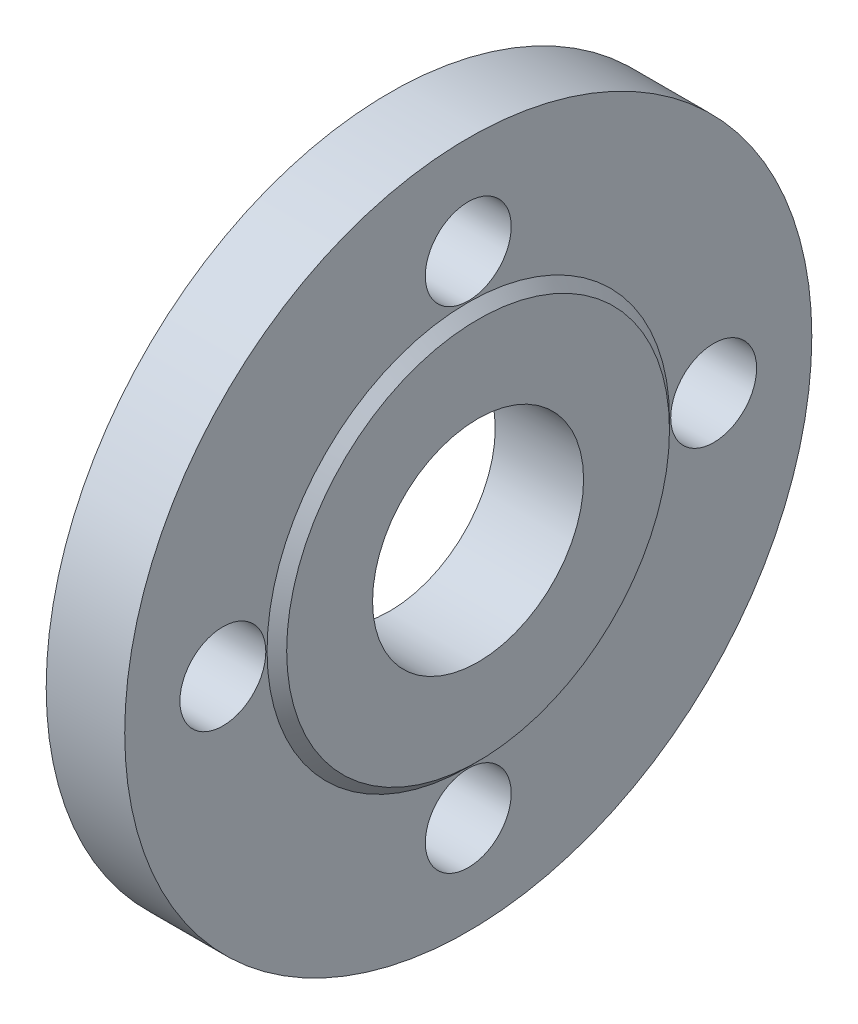
from build123d import *

# Parameters (mm, degrees)
CUT_EXTRUDE_1_DEPTH      = 101.279609094
CUT_EXTRUDE_1_DEPTH_BACK = 101.279609094
SKETCH_2_R               = 8.75


with BuildPart() as part:
    # 草图1 → 旋转1 (revolve)
    with BuildSketch(Plane(origin=(0, 0, 0), x_dir=(1, 0, 0), z_dir=(0, 1, 0)), mode=Mode.PRIVATE) as revolve_1_sk:
        Polygon((0, 21.5), (0, 70), (16, 70), (16, 41), (18, 39), (18, 21.5), align=None)
    revolve(revolve_1_sk.sketch.rotate(Axis((0, 0, 0), (1, 0, 0)), 180), axis=Axis((0, 0, 0), (1, 0, 0)))

    # 草图2 → 切除-拉伸1 (cut, two sides: drawn at the far end of the back side and taken through both)
    with BuildSketch(Plane(origin=(16, 0, 0), x_dir=(0, 0, -1), z_dir=(1, 0, 0)).offset(-CUT_EXTRUDE_1_DEPTH_BACK)):
        with Locations((0, 50)):
            Circle(SKETCH_2_R)
        with Locations((50, 0)):
            Circle(SKETCH_2_R)
        with Locations((0, -50)):
            Circle(SKETCH_2_R)
        with Locations((-50, 0)):
            Circle(SKETCH_2_R)
    extrude(amount=CUT_EXTRUDE_1_DEPTH + CUT_EXTRUDE_1_DEPTH_BACK, mode=Mode.SUBTRACT)


solid = part.part
